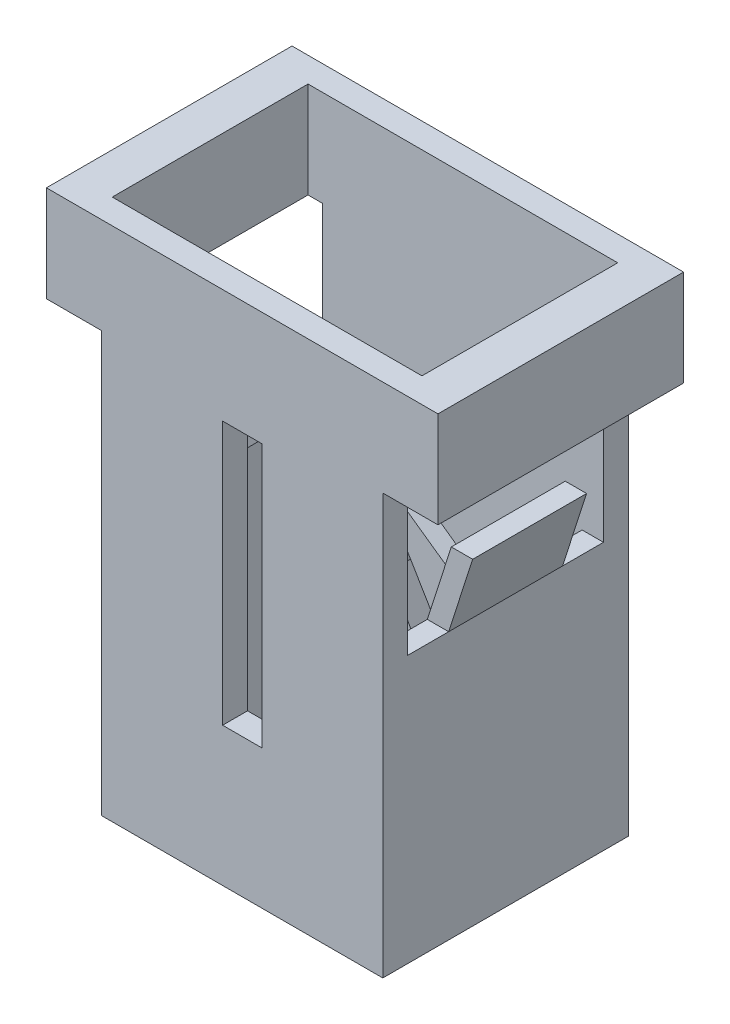
SolidWorks part; units mm, degrees
ref_plane "前视基准面" through (0, 0, 0) normal (0, 0, 1) x (1, 0, 0)
ref_plane "上视基准面" through (0, 0, 0) normal (0, 1, 0) x (1, 0, 0)
ref_plane "右视基准面" through (0, 0, 0) normal (1, 0, 0) x (0, 0, -1)
sketch "草图1" plane through (0, 0, 0) normal (0, 0, 1) x (1, 0, 0)
  line L0 (-3.95, 0) -> (3.95, 0)
  line L1 (3.95, 0) -> (3.95, 12.3)
  line L5 (3.95, 12.3) -> (5.5, 12.3)
  line L6 (5.5, 12.3) -> (5.5, 15)
  line L7 (5.5, 15) -> (-5.5, 15)
  line L8 (-5.5, 15) -> (-5.5, 12.3)
  line L9 (-5.5, 12.3) -> (-3.95, 12.3)
  line L13 (-3.95, 12.3) -> (-3.95, 0)
  dimension "D1" = 7.9
  dimension "D2" = 3.95
  dimension "D7" = 15
  dimension "D10" = 2.7
  dimension "D11" = 2.7
  dimension "D15" = 11
  dimension "D16" = 5.5
extrude "凸台-拉伸1" add sketch "草图1" along normal mid plane 6.9
chamfer "倒角1" distance 0.5 angle 45 4 edges at (-3.95, 0, 0) (0, 0, 3.45) (3.95, 0, 0) (0, 0, -3.45)
sketch "草图2" plane through (-3.95, 0, 0) normal (-1, 0, 0) x (0, 0, 1)
  line L0 (3.45, 12.3) -> (-3.45, 12.3) construction
  line L1 (-2.75, 12.3) -> (2.75, 12.3)
  line L2 (-2.75, 12.3) -> (-2.75, 8)
  line L3 (-2.75, 8) -> (2.75, 8)
  line L4 (2.75, 12.3) -> (2.75, 8)
  line L5 (2.95, 0) -> (-2.95, 0) construction
  dimension "D1" = 8
  dimension "D2" = 5.5
  dimension "D3" = 2.75
extrude "切除-拉伸1" cut sketch "草图2" against normal through all
sketch "草图3" plane through (0, 15, 0) normal (0, 1, 0) x (1, 0, 0)
  line L1 (-4.35, 2.75) -> (4.35, 2.75)
  line L2 (-4.35, 2.75) -> (-4.35, -2.75)
  line L3 (-4.35, -2.75) -> (4.35, -2.75)
  line L4 (4.35, 2.75) -> (4.35, -2.75)
  dimension "D1" = 8.7
  dimension "D2" = 4.35
  dimension "D3" = 5.5
  dimension "D4" = 2.75
extrude "切除-拉伸2" cut sketch "草图3" against normal up to surface (2.7 mm away) up to face at (0, 12.3, 0)
sketch "草图5" plane through (0, 15, 0) normal (0, 1, 0) x (1, 0, 0)
  line L1 (-3.35, 2.75) -> (3.35, 2.75)
  line L2 (-3.35, 2.75) -> (-3.35, -2.75)
  line L3 (-3.35, -2.75) -> (3.35, -2.75)
  line L4 (3.35, 2.75) -> (3.35, -2.75)
  line L6 (-3.95, 2.75) -> (-3.95, -2.75) construction
  line L7 (3.95, 2.75) -> (3.95, -2.75) construction
  line L8 (4.35, 2.75) -> (-4.35, 2.75) construction
  line L9 (-4.35, -2.75) -> (4.35, -2.75) construction
  dimension "D1" = 0.6
  dimension "D2" = 0.6
extrude "切除-拉伸3" cut sketch "草图5" against normal blind 14
sketch "草图6" plane through (0, 0, 3.45) normal (0, 0, 1) x (1, 0, 0)
  line L0 (5.5, 15) -> (-5.5, 15) construction
  line L1 (-0.55, 11.8) -> (0.55, 11.8)
  line L2 (-0.55, 11.8) -> (-0.55, 4.4)
  line L3 (-0.55, 4.4) -> (0.55, 4.4)
  line L4 (0.55, 11.8) -> (0.55, 4.4)
  line L5 (-0.55, 11.8) -> (0.55, 4.4) construction
  line L6 (-0.55, 4.4) -> (0.55, 11.8) construction
  point P0 (0, 8.1)
  dimension "D1" = 1.1
  dimension "D2" = 7.4
  dimension "D3" = 3.2
extrude "切除-拉伸4" cut sketch "草图6" against normal blind 1
sketch "草图7" plane through (0, 0, 0) normal (0, 0, 1) x (1, 0, 0)
  line L0 (-3.95, 8) -> (-4.625, 10.1)
  line L1 (-4.625, 10.1) -> (-4.025, 10.1)
  line L2 (-4.025, 10.1) -> (-3.35, 8)
  line L3 (-3.35, 8) -> (-3.95, 8)
  line L4 (0, -0.7915) -> (0, 16.3286) construction
  line L5 (-5.5, 12.3) -> (-3.95, 12.3) construction
  line L6 (3.35, 8) -> (3.95, 8)
  line L7 (4.025, 10.1) -> (3.35, 8)
  line L8 (4.625, 10.1) -> (4.025, 10.1)
  line L9 (3.95, 8) -> (4.625, 10.1)
  dimension "D1" = 2.2
  dimension "D2" = 4.625
extrude "凸台-拉伸2" add sketch "草图7" along normal mid plane 3.2
sketch "草图8" plane through (0, 0, 0) normal (0, -1, 0) x (1, 0, 0)
  line L1 (-2.55, -1.25) -> (-0.55, -1.25)
  line L2 (-2.55, -1.25) -> (-2.55, -2.25)
  line L3 (-2.55, -2.25) -> (-0.55, -2.25)
  line L4 (-0.55, -1.25) -> (-0.55, -2.25)
  line L5 (0.55, -1.25) -> (2.55, -1.25)
  line L6 (0.55, -1.25) -> (0.55, -2.25)
  line L7 (0.55, -2.25) -> (2.55, -2.25)
  line L8 (2.55, -1.25) -> (2.55, -2.25)
  line L9 (3.95, -3.45) -> (-3.95, -3.45) construction
  dimension "D1" = 2
  dimension "D2" = 2
  dimension "D3" = 0.55
  dimension "D4" = 1.1
  dimension "D5" = 1
  dimension "D6" = 1
  dimension "D7" = 1.2
extrude "切除-拉伸5" cut sketch "草图8" against normal blind 3.5
sketch "草图9" plane through (0, 1, 0) normal (0, 1, 0) x (1, 0, 0)
  line L0 (5.5, 3.45) -> (-5.5, 3.45) construction
  circle A0 centre (0, -0.55) radius 0.75
  dimension "D1" = 1.5
  dimension "D2" = 4
extrude "凸台-拉伸3" add sketch "草图9" along normal blind 3.2
draft "拔模1" type of draft neutral plane draft angle 2 faces to draft 1 face at (0, 4.2, 1.3) neutral plane through (0, 1, 0) neutral plane normal (0, 1, 0) parameters "D1"=2
sketch "草图10" plane through (0, 0, -3.45) normal (0, 0, -1) x (-1, 0, 0)
  line L0 (-2.05, 4.3) -> (-2.05, 2.7)
  line L1 (-2.05, 2.7) -> (-1.15, 3.1)
  line L2 (-1.15, 3.1) -> (-0.2, 2.4)
  line L3 (-0.2, 2.4) -> (1.05, 2.4)
  line L4 (1.05, 2.4) -> (2.05, 4.3)
  line L5 (2.05, 4.3) -> (2.05, 7.2)
  line L6 (2.05, 7.2) -> (0.15, 4)
  line L7 (-0.55, 4.6) -> (0.15, 4)
  line L8 (-0.55, 4.6) -> (-2.05, 4.3)
  line L9 (-3.95, 0.5) -> (-3.95, 12.3) construction
  line L10 (3.95, 12.3) -> (3.95, 0.5) construction
  line L11 (3.45, 0) -> (-3.45, 0) construction
  point P2 (-2.05, 3.5)
  dimension "D1" = 1.9
  dimension "D2" = 1.9
  dimension "D3" = 2.4
  dimension "D4" = 3.1
  dimension "D5" = 4.3
  dimension "D6" = 2.7
  dimension "D7" = 4.3
  dimension "D8" = 7.2
  dimension "D9" = 4
  dimension "D10" = 4.6
  dimension "D11" = 2.8
  dimension "D12" = 3.75
  dimension "D13" = 5
  dimension "D14" = 3.4
  dimension "D15" = 4.1
extrude "切除-拉伸6" cut sketch "草图10" against normal blind 3.2
sketch "草图11" plane through (0, 0, -2.75) normal (0, 0, 1) x (1, 0, 0)
  line L0 (0.55, 4.6) -> (2.05, 4.3) construction
  line L1 (-0.15, 4) -> (0.55, 4.6) construction
  line L2 (-2.05, 7.2) -> (-0.15, 4) construction
  line L3 (0.55, 4.6) -> (2.05, 4.3)
  line L4 (-0.15, 4) -> (0.55, 4.6)
  line L5 (-2.05, 7.2) -> (-0.15, 4)
  line L6 (-2.05, 7.2) -> (2.05, 4.3)
extrude "凸台-拉伸4" add sketch "草图11" along normal blind 0.5
scale "缩放比例1" scale about centroid uniform scaling yes scale factor 0.7
